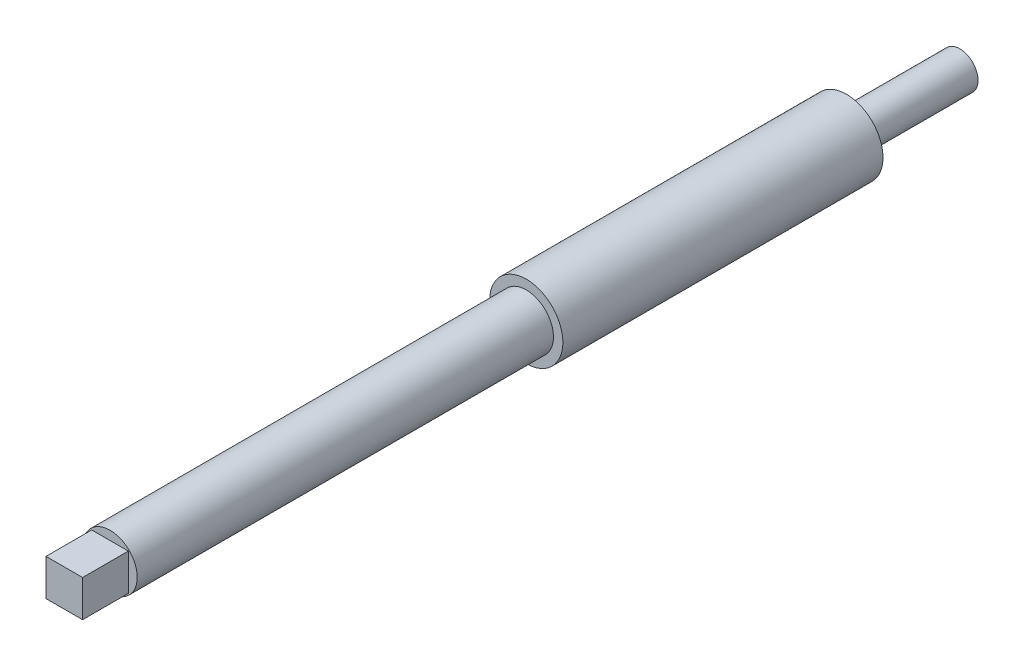
from build123d import *

# Parameters (mm, degrees)
SKETCH_1_R      = 5.95
EXTRUDE_1_DEPTH = 91
SKETCH_2_W      = 8
SKETCH_2_H      = 8
EXTRUDE_2_DEPTH = 10
SKETCH_3_R      = 8
EXTRUDE_3_DEPTH = 70
SKETCH_4_R      = 4
EXTRUDE_4_DEPTH = 25


with BuildPart() as part:
    # 草图1 → 凸台-拉伸1 (new body)
    with BuildSketch(Plane.XY):
        Circle(SKETCH_1_R)
    extrude(amount=EXTRUDE_1_DEPTH)

    # 草图2 → 凸台-拉伸2 (add)
    with BuildSketch(Plane.XY.offset(91)):
        Rectangle(SKETCH_2_W, SKETCH_2_H)
    extrude(amount=EXTRUDE_2_DEPTH)

    # 草图3 → 凸台-拉伸3 (add)
    with BuildSketch(Plane(origin=(0, 0, 0), x_dir=(-1, 0, 0), z_dir=(0, 0, -1))):
        Circle(SKETCH_3_R)
    extrude(amount=EXTRUDE_3_DEPTH)

    # 草图4 → 凸台-拉伸4 (add)
    with BuildSketch(Plane(origin=(0, 0, -70), x_dir=(-1, 0, 0), z_dir=(0, 0, -1))):
        with Locations((0.224619263, 0)):
            Circle(SKETCH_4_R)
    extrude(amount=EXTRUDE_4_DEPTH)


solid = part.part
